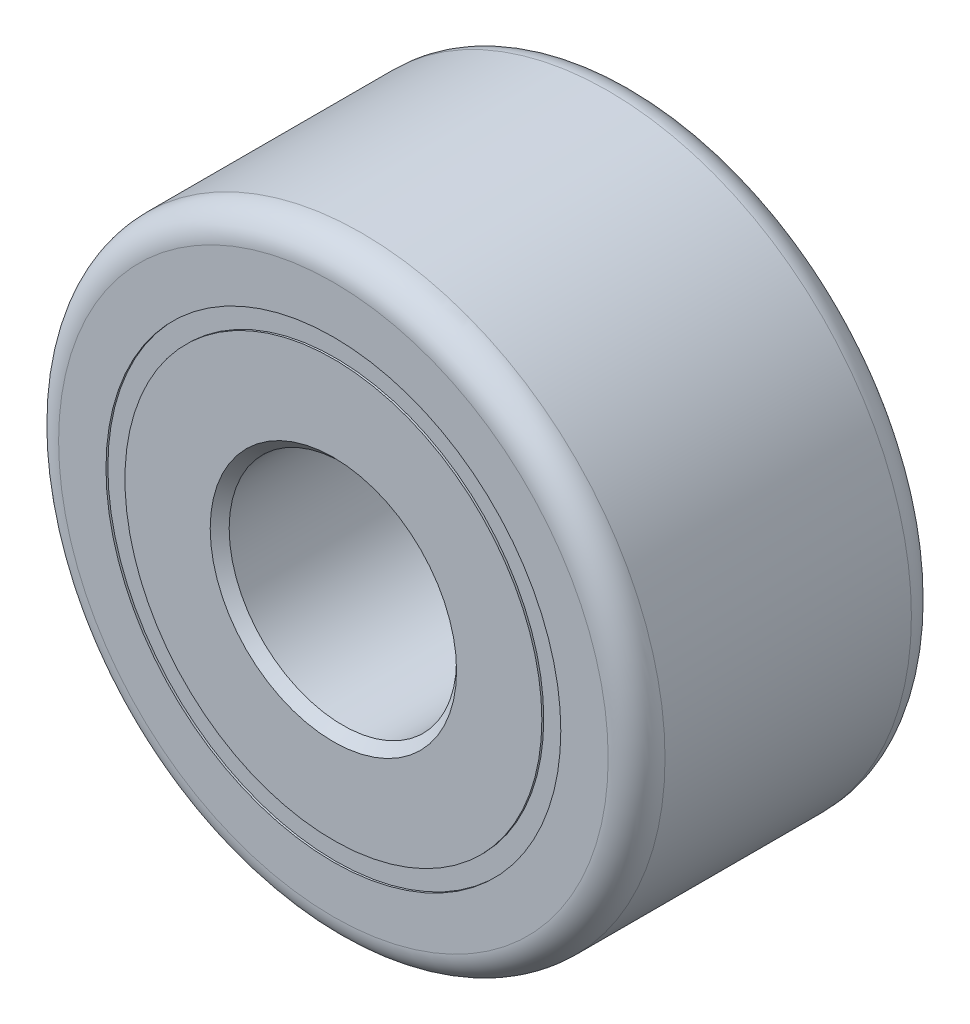
SolidWorks part; units mm, degrees
ref_plane "Front Plane" through (0, 0, 0) normal (0, 0, 1) x (1, 0, 0)
ref_plane "Top Plane" through (0, 0, 0) normal (0, 1, 0) x (1, 0, 0)
ref_plane "Right Plane" through (0, 0, 0) normal (1, 0, 0) x (0, 0, -1)
sketch "Sketch1" plane through (0, 0, 0) normal (0, 0, 1) x (1, 0, 0)
  circle A0 centre (0, 0) radius 16
  dimension "D1" = 32
extrude "Boss-Extrude1" add sketch "Sketch1" along normal blind 16
sketch "Sketch2" plane through (0, 0, 16) normal (0, 0, 1) x (1, 0, 0)
  circle A0 centre (0, 0) radius 6
  dimension "D1" = 12
extrude "Cut-Extrude1" cut sketch "Sketch2" against normal blind 16
sketch "Sketch3" plane through (0, 0, 16) normal (0, 0, 1) x (1, 0, 0)
  circle A0 centre (0, 0) radius 12
  circle A1 centre (0, 0) radius 11
  dimension "D1" = 22
  dimension "D2" = 24
extrude "Cut-Extrude2" cut sketch "Sketch3" against normal blind 0.1
fillet "Fillet1" radius 1.5 2 edges at (16, 0, 0) (16, 0, 16)
chamfer "Chamfer1" distance 0.5 angle 45 2 edges at (6, 0, 0) (6, 0, 16)
